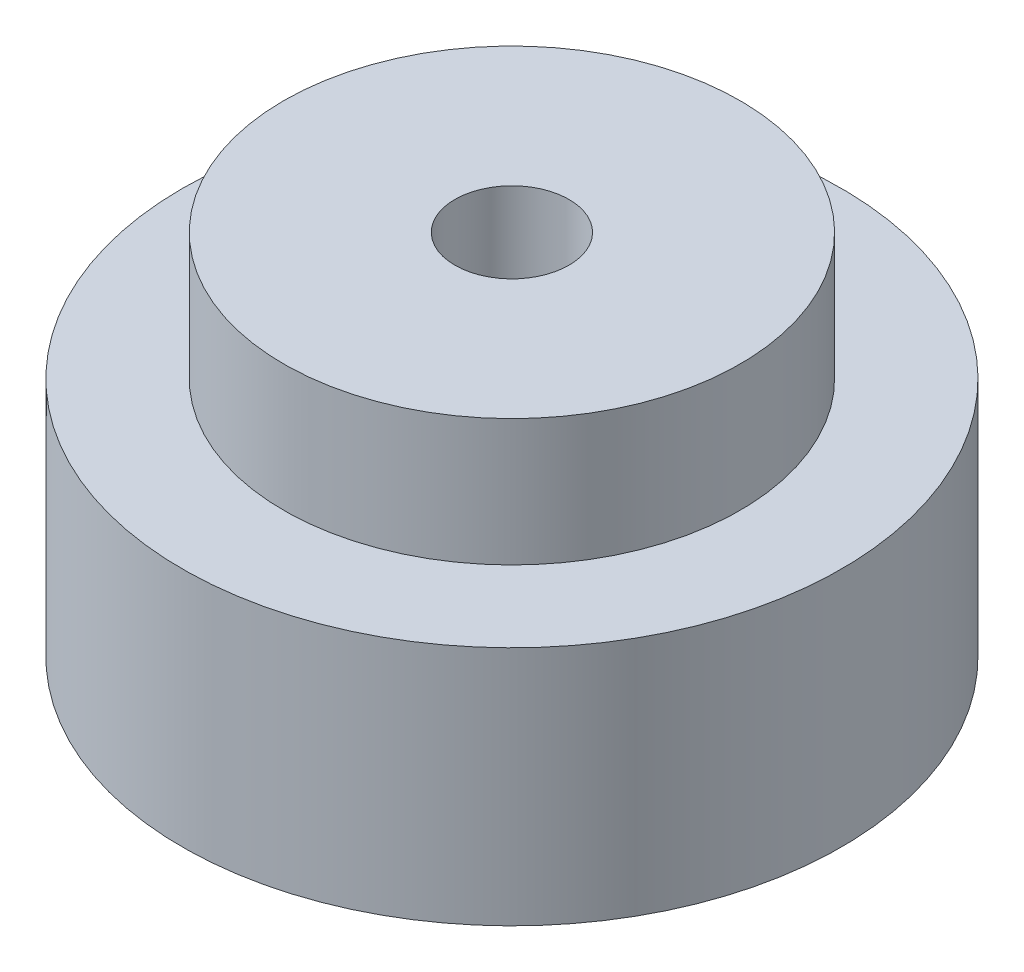
from build123d import *

# Parameters (mm, degrees)
M10X1_0_1_D         = 9
SKETCH_4_R          = 3
CUT_EXTRUDE_1_DEPTH = 47.829477896


with BuildPart() as part:
    # 草图1 → 旋转1 (revolve)
    with BuildSketch(Plane.XY, mode=Mode.PRIVATE) as revolve_1_sk:
        Polygon((20, 0), (26, 0), (26, 19), (18, 19), (18, 29), (0, 29), (0, 17), (5, 17), (20, 11), align=None)
    revolve(revolve_1_sk.sketch.rotate(Axis((0, 29.712230849, 0), (0, -1, 0)), 180), axis=Axis((0, 29.712230849, 0), (0, -1, 0)))

    # M10x1.0 螺纹孔1 (through all)
    with Locations(Plane(origin=(0, 29, 0), x_dir=(1, 0, 0), z_dir=(0, 1, 0))):
        with Locations((0, 0)):
            Hole(M10X1_0_1_D / 2)

    # 草图4 → 切除-拉伸1 (cut, through all)
    with BuildSketch(Plane(origin=(0, 0, 0), x_dir=(0, 0, -1), z_dir=(1, 0, 0))):
        with Locations(Location((0, 9, 0), (0, 0, 270.000000001))):
            Circle(SKETCH_4_R)
    extrude(amount=-CUT_EXTRUDE_1_DEPTH, mode=Mode.SUBTRACT)


solid = part.part
